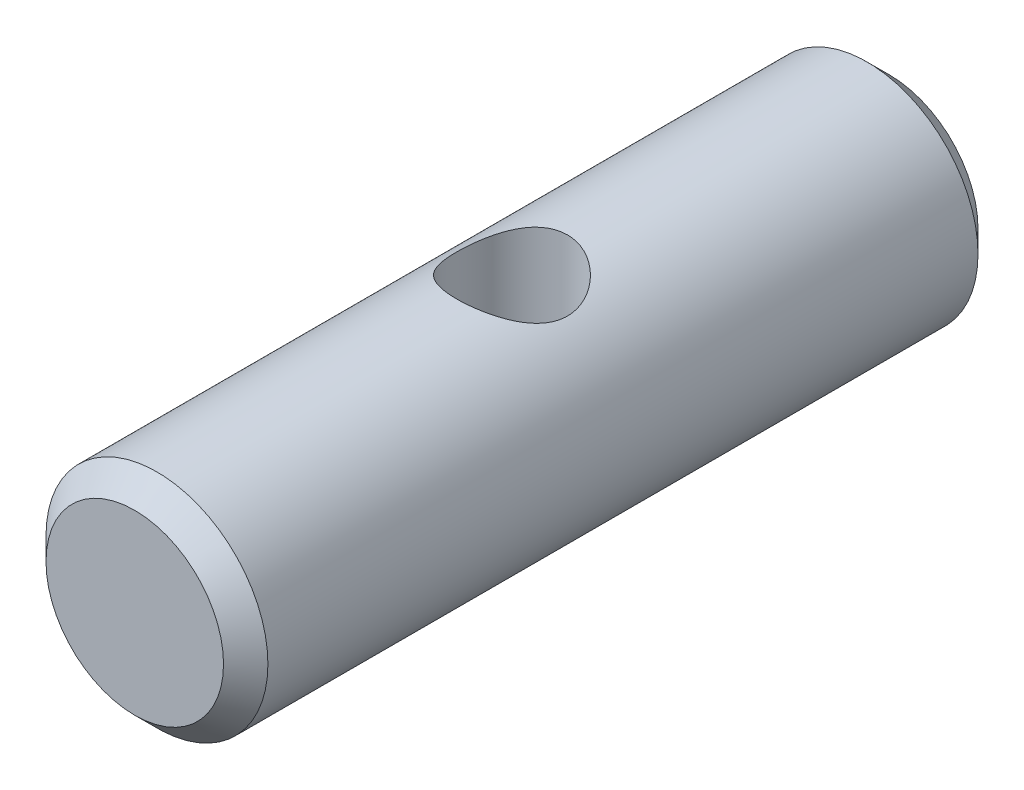
SolidWorks part; units mm, degrees
ref_plane "Front Plane" through (0, 0, 0) normal (0, 0, 1) x (1, 0, 0)
ref_plane "Top Plane" through (0, 0, 0) normal (0, 1, 0) x (1, 0, 0)
ref_plane "Right Plane" through (0, 0, 0) normal (1, 0, 0) x (0, 0, -1)
other "Configuration Table"
ref_plane "Plane1" through (0, 0, 0) normal (0, -1, 0) x (1, 0, 0)
sketch "Sketch1" plane through (0, 0, 0) normal (0, -1, 0) x (1, 0, 0)
  line L0 (5, 34) -> (0, 34)
  line L1 (0, 34) -> (0, 0)
  line L2 (0, 0) -> (5, 0)
  line L3 (5, 0) -> (5, 34)
  line L4 (0, 34) -> (0, 0) construction
revolve "Revolve1" add sketch "Sketch1" angle 360 about L4
hole_wizard "Ø5.0 (5) Diameter Hole1" positions "3DSketch1" profile "Sketch2" hole size "Ø5.0" standard "ANSI Metric"
sketch3d "3DSketch1"
  point P0 (0, -5, 17)
sketch "Sketch2" plane through (0, -5, 17) normal (1, 0, 0) x (0, 0, -1)
  line L0 (0, 0) -> (0, 10)
  line L1 (0, 10) -> (2.5, 10)
  line L2 (2.5, 10) -> (2.5, 0)
  line L5 (2.5, 0) -> (0, 0)
  line L11 (0, -6.35) -> (0, 107.95) construction
  dimension "通孔孔直径" = 5
  dimension "通孔孔深度" = 10
chamfer "Chamfer1" distance 1 angle 45 2 edges at (-5, 0, 34) (-5, 0, 0)
